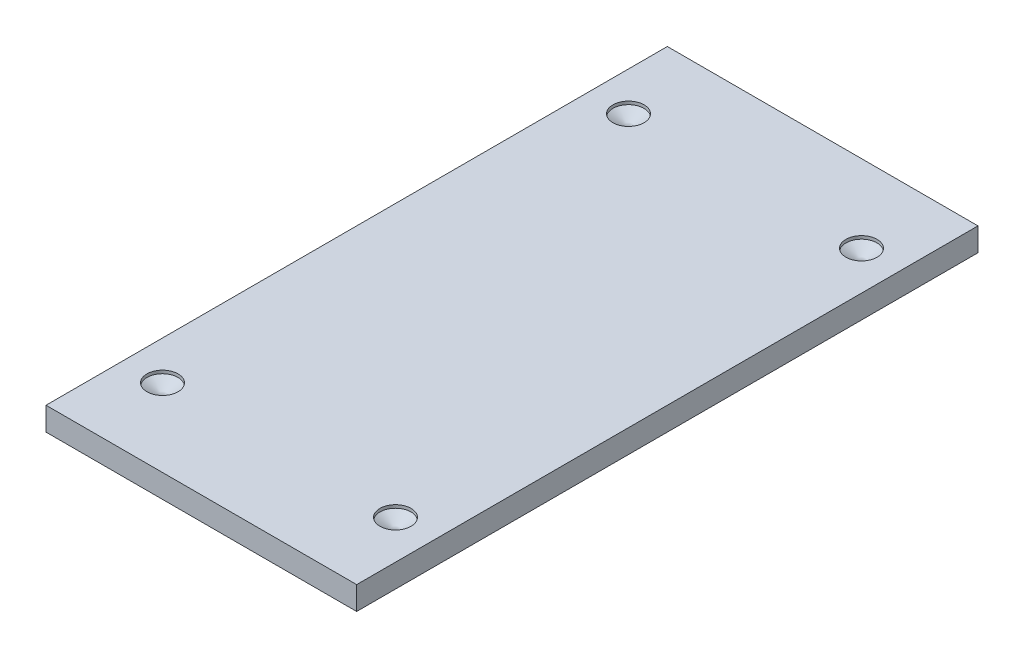
from build123d import *

# Parameters (mm, degrees)
SKETCH1_W                      = 200
SKETCH1_H                      = 400
BOSS_EXTRUDE1_DEPTH            = 15
F_20_0_20_DIAMETER_HOLE1_D     = 20
F_20_0_20_DIAMETER_HOLE1_DEPTH = 2
F_20_0_20_DIAMETER_HOLE1_TIP   = 6.00860619


with BuildPart() as part:
    # Sketch1 → Boss-Extrude1 (new body)
    with BuildSketch(Plane(origin=(0, 0, 0), x_dir=(1, 0, 0), z_dir=(0, 1, 0))):
        Rectangle(SKETCH1_W, SKETCH1_H)
    extrude(amount=BOSS_EXTRUDE1_DEPTH)

    # Ø20.0 (20) Diameter Hole1
    with Locations(Plane(origin=(0, 15, 0), x_dir=(1, 0, 0), z_dir=(0, 1, 0))):
        with Locations((-75, 150), (-75, -150), (75, -150), (75, 150)):
            Hole(F_20_0_20_DIAMETER_HOLE1_D / 2, depth=F_20_0_20_DIAMETER_HOLE1_DEPTH)
            with Locations((0, 0, -(F_20_0_20_DIAMETER_HOLE1_DEPTH + F_20_0_20_DIAMETER_HOLE1_TIP / 2))):  # 118° drill point
                Cone(0, F_20_0_20_DIAMETER_HOLE1_D / 2, F_20_0_20_DIAMETER_HOLE1_TIP, mode=Mode.SUBTRACT)


solid = part.part
